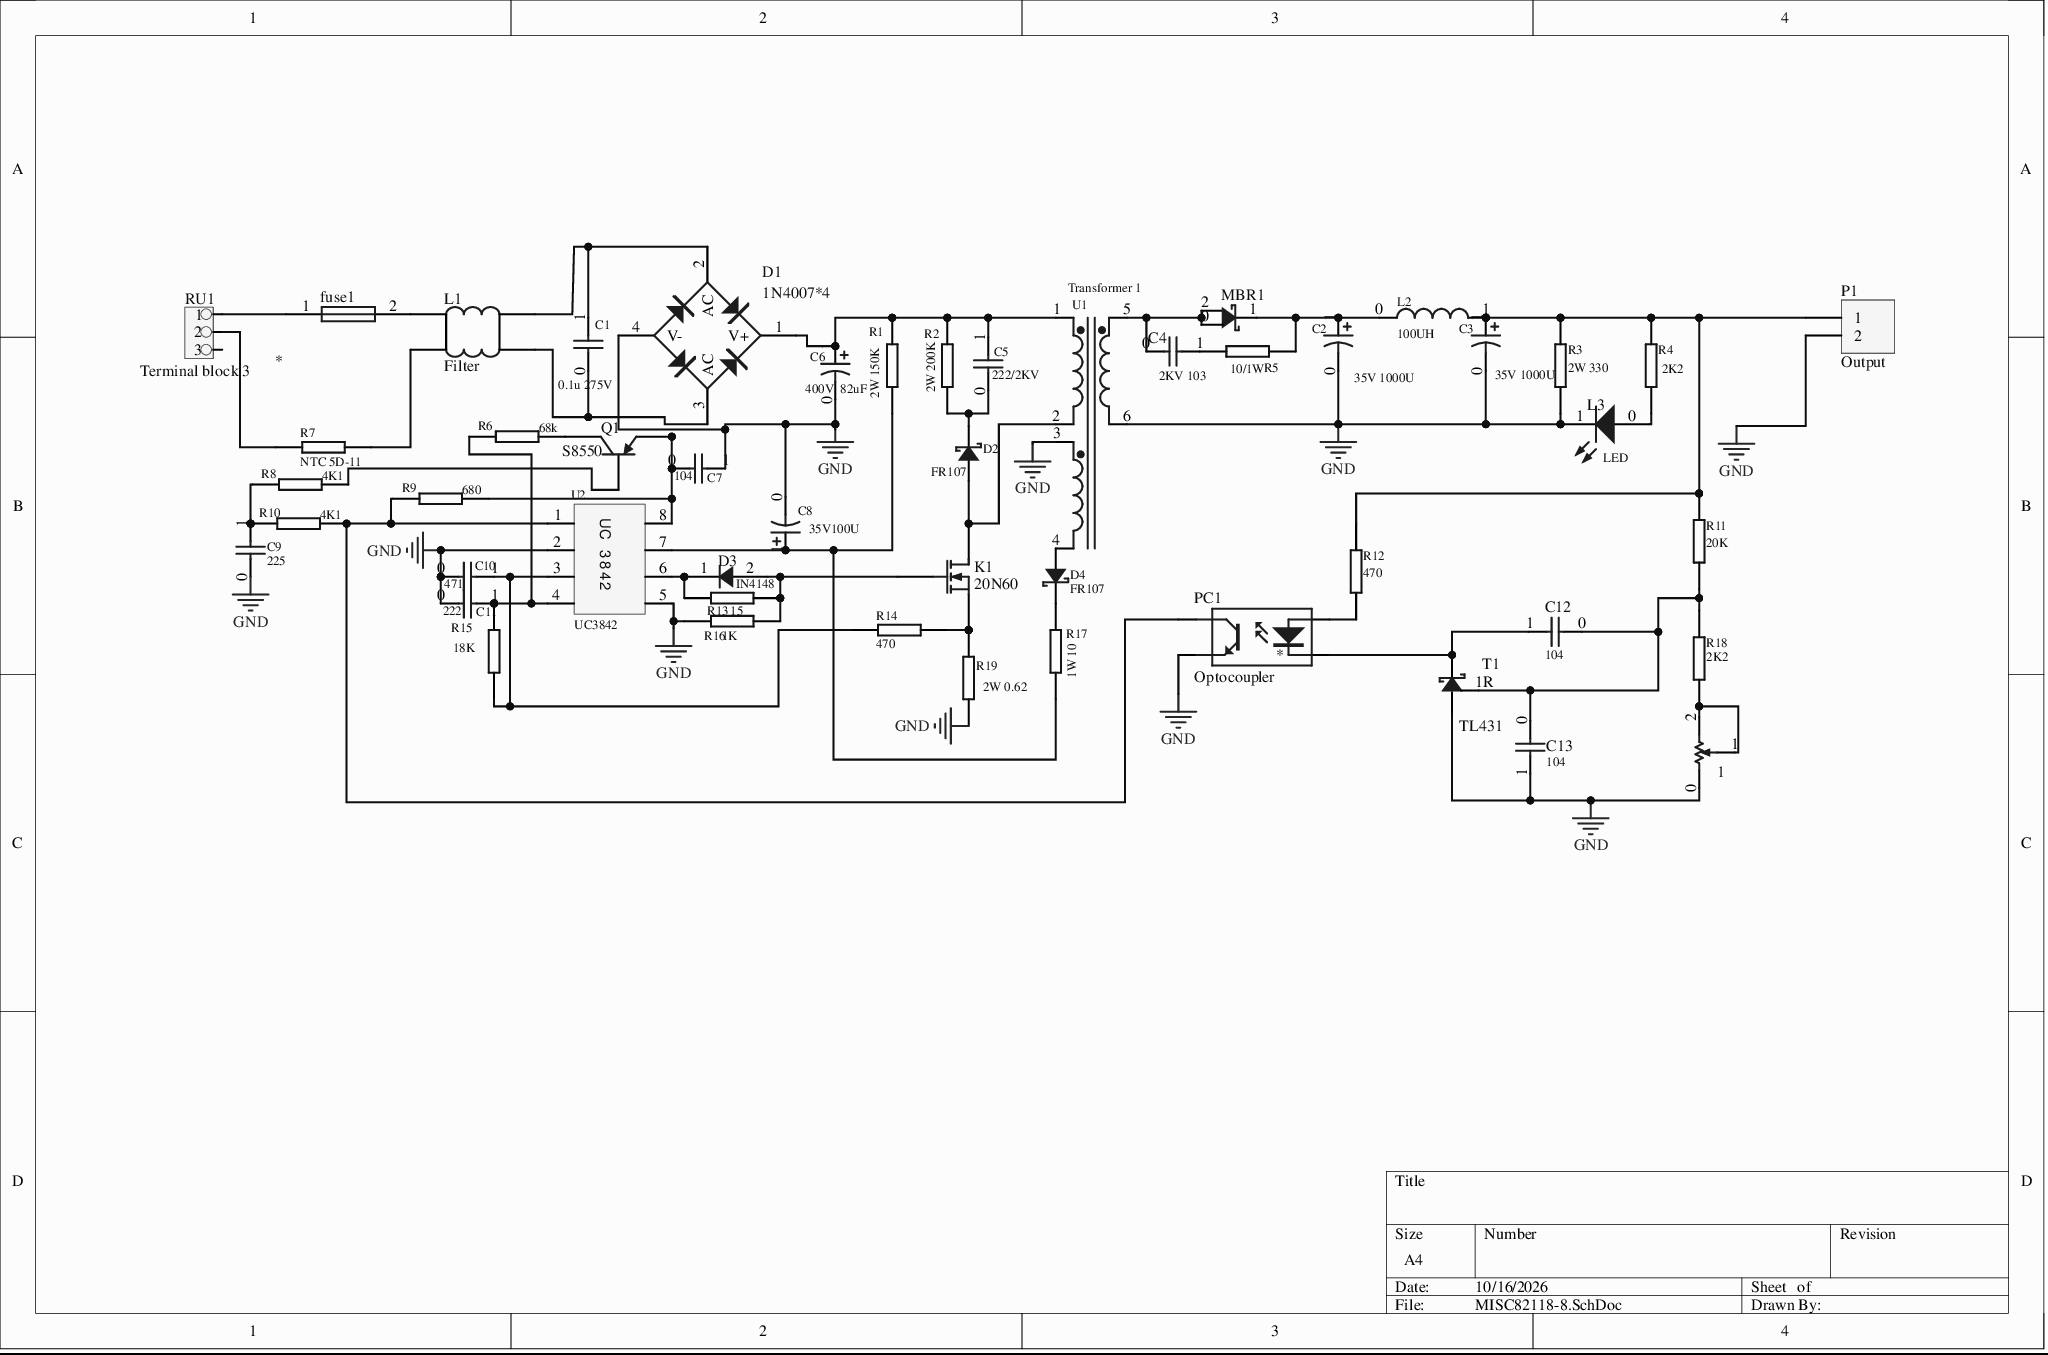
[diagram p0: MISC82118-8.SchDoc]
# Altium project MISC82118-6.PrjPcb
1 sheet, 50 parts. Net scope: global (net labels, ports and power ports of the same name join across sheets).
Board file: MISC82118.PcbDoc

## Sheet MISC82118-8.SchDoc
size A4

### Parts
1  (no value)  [VR5]
C1  0.1u 275V  [RAD-0.1]
C2  35V 1000U  [RB7.6-15]
C3  35V 1000U  [RB7.6-15]
C4  2KV 103  [RAD-0.1]
C5  222/2KV  [RAD-0.1]
C6  400V  82uF  [RB7.6-15]
C7  104  [RAD-0.1]
C8  35V100U  [RB7.6-15]
C9  225  [RAD-0.1]
C10  471  [RAD-0.1]
C11  222  [RAD-0.1]
C12  104  [RAD-0.1]
C13  104  [RAD-0.1]
D1  1N4007*4  [D-38]
D2  FR107  [DO-35]
D3  IN4148  [DO-35]
D4  FR107  [DO-35]
fuse1  (no value)  [PIN-W2/E2.8]
K1  20N60  [E3]
L1  Filter  [TRANS]
L2  100UH  [AL0204]
L3  LED  [LED3MM]
MBR1  (no value)  [TO-262-AA]
P1  Output  [HDR1X2]
PC1  *  [DIP-4]
Q1  S8550  [TO-92A]
R1  2W 150K  [J1-0603]
R2  2W 200K  [J1-0603]
R3  2W 330  [J1-0603]
R4  2K2  [J1-0603]
R5  10/1W  [J1-0603]
R6  68k  [J1-0603]
R7  NTC 5D-11  [6-0805_N]
R8  4K1  [J1-0603]
R9  680  [J1-0603]
R10  4K1  [J1-0603]
R11  20K  [J1-0603]
R12  470  [J1-0603]
R13  15  [J1-0603]
R14  470  [J1-0603]
R15  18K  [J1-0603]
R16  1K  [J1-0603]
R17  1W 10  [J1-0603]
R18  2K2  [J1-0603]
R19  2W 0.62  [J1-0603]
RU1  *  Comm: Terminal block 3  [KF2510-3P]
T1  TL431  [TO-262-AA]
U1  Transformer 1  [TRF_6]
U2  UC3842  [DIP-8]

### Nets
GND: 1.0 C2.0 C3.0 C6.0 C7.1 C8.0 C9.0 C10.0 C11.0 C13.1 D1.4(V-) L3.1 P1.2 PC1.4 R3.0 R16.0 R19.0 T1.2A U1.3 U1.6 U2.2 U2.5
Net1_1: 1.1 1.2 R18.1
NetC1_0: C1.0 D1.3(AC) L1.3
NetC1_1: C1.1 D1.2(AC) L1.2
NetC2_1: C2.1 L2.0 MBR1.1 R5.1
NetC3_1: C3.1 L2.1 P1.1 R3.1 R4.1 R11.1 R12.0
NetC4_0: C4.0 MBR1.0 MBR1.2 U1.5
NetC4_1: C4.1 R5.0
NetC5_0: C5.0 D2.1 R2.0
NetC5_1: C5.1 C6.1 D1.1(V+) R1.1 R2.1 U1.1
NetC7_0: C7.0 Q1.1(E) R9.1 U2.8
NetC8_1: C8.1 R1.0 R17.0 U2.7
NetC9_1: C9.1 R8.0 R10.0
NetC10_1: C10.1 R14.0 R15.0 U2.3
NetC11_1: C11.1 R6.0 R15.1 U2.4
NetC12_0: C12.0 C13.0 R11.0 R18.0 T1.1R
NetC12_1: C12.1 PC1.2 T1.3K
NetD2_2: D2.2 K1.2D U1.2
NetD3_1: D3.1 R13.0 U2.6
NetD3_2: D3.2 K1.1G R13.1 R16.1
NetD4_1: D4.1 R17.1
NetD4_2: D4.2 U1.4
Netfuse1_1: fuse1.1 RU1.1
Netfuse1_2: fuse1.2 L1.1
NetK1_3S: K1.3S R14.1 R19.1
NetL1_4: L1.4 R7.0
NetL3_0: L3.0 R4.0
NetPC1_1: PC1.1 R12.1
NetPC1_3: PC1.3 R9.0 R10.1 U2.1
NetQ1_2: Q1.2(B) R8.1
NetQ1_3: Q1.3(C) R6.1
NetR7_1: R7.1 RU1.2

Not connected (* = marked no-connect by the designer): RU1 3

### Library data of the parts
1 = 三角电位器
C1 C4 C5 C7 C9-C13 = 电容
C2 C3 C6 C8 = 电解电容1
D1 = BRIDGE1: Diode Bridge
D2 D4 = 肖特基二极管
D3 = 二极管
fuse1 = 保险丝
K1 = N-MOS
L1 = 滤波器
L2 = 电感
L3 = 发光二极管
MBR1 = 肖特基二极管2
P1 = Header 2: Header, 2-Pin; LatestRevisionDate: 17-Jul-2002; LatestRevisionNote: Re-released for DXP Platform.; Publisher: Altium Limited
PC1 = 光电耦合器
Q1 = 2N3906: PNP General Purpose Amplifier; Published: 8-Jun-2000; LatestRevisionDate: 15-Jan-2003; LatestRevisionNote: PCB Footprint 'BCY-W3/D4.7' replaced; DatasheetVersion: 1997; PackageVersion: Sep-1998; PackageReference: TO-92A; Code_JEDEC: TO-92A; ComponentLink1Description: Manufacturer Link; ComponentLink2Description: Datasheet; ComponentLink2URL: example.com/ds/2N%2F2N3906.pdf; Publisher: Altium Limited
R1-R19 = 电阻
RU1 = 接线端子3
U1 = 变压器1